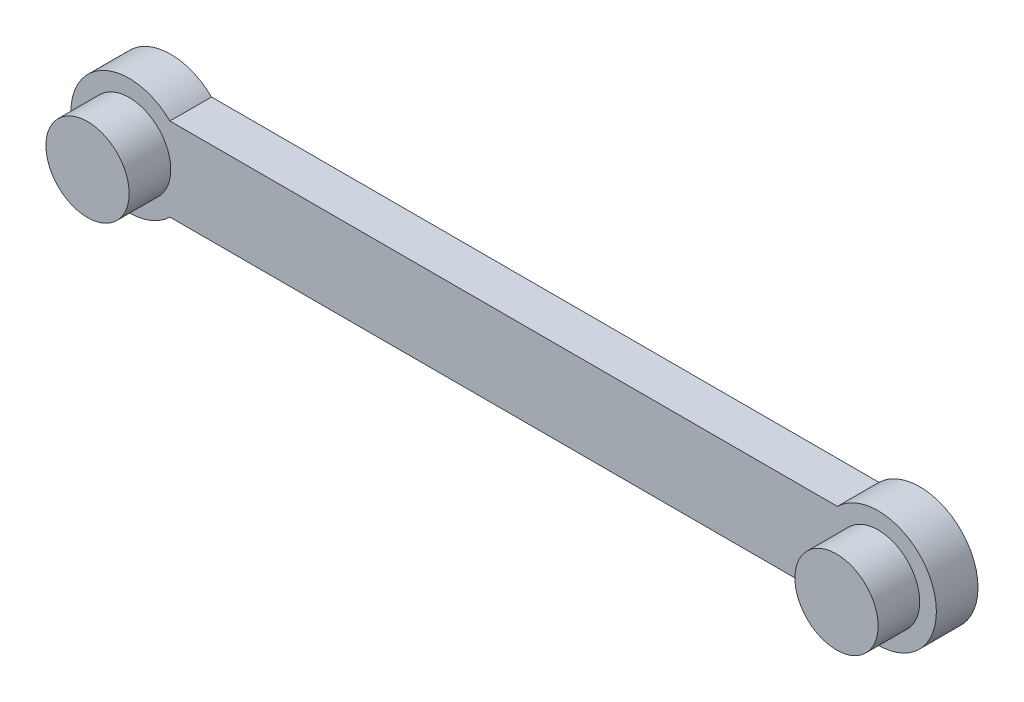
SolidWorks part; units mm, degrees
ref_plane "Plane1" through (0, 0, 0) normal (0, 0, 1) x (1, 0, 0)
ref_plane "Plane2" through (0, 0, 0) normal (0, 1, 0) x (1, 0, 0)
ref_plane "Plane3" through (0, 0, 0) normal (1, 0, 0) x (0, 0, -1)
sketch "Sketch1" plane through (0, 0, 0) normal (0, 0, 1) x (1, 0, 0)
  line L0 (0, 0) -> (90, 0) construction
  line L1 (4.899, -5) -> (85.101, -5)
  line L2 (4.899, 5) -> (85.101, 5)
  arc A0 (4.899, 5) -> (4.899, -5) centre (0, 0) ccw
  arc A1 (85.101, -5) -> (85.101, 5) centre (90, 0) ccw
  dimension "D2" = 7
  dimension "D3" = 7
  dimension "D1" = 90
  dimension "D4" = 10
extrude "Base-Extrude" add sketch "Sketch1" along normal blind 5
sketch "Sketch2" plane through (0, 0, 5) normal (0, 0, 1) x (1, 0, 0)
  circle A0 centre (0, 0) radius 5
  circle A1 centre (90, 0) radius 5
  dimension "D1" = 10
  dimension "D2" = 10
extrude "Boss-Extrude1" add sketch "Sketch2" along normal blind 5
